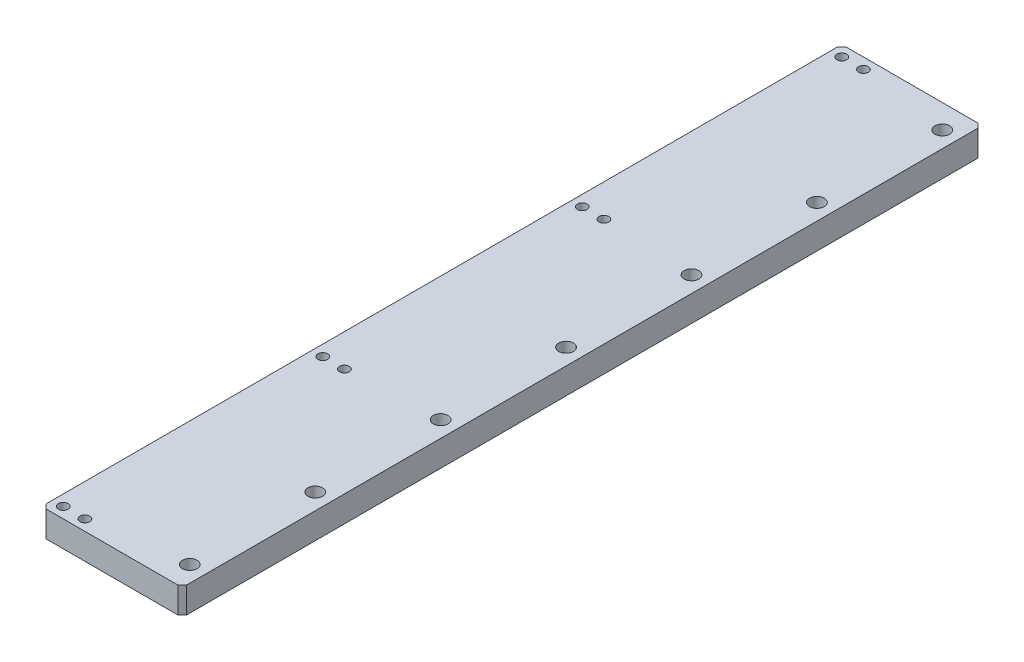
SolidWorks part; units mm, degrees
material "A6061"
ref_plane "前基準面" through (0, 0, 0) normal (0, 0, 1) x (1, 0, 0)
ref_plane "上基準面" through (0, 0, 0) normal (0, 1, 0) x (1, 0, 0)
ref_plane "右基準面" through (0, 0, 0) normal (1, 0, 0) x (0, 0, -1)
sketch "草图1" plane through (0, 0, 0) normal (0, 1, 0) x (1, 0, 0)
  line L1 (-32.5, 185) -> (32.5, 185)
  line L2 (-32.5, 185) -> (-32.5, -185)
  line L3 (-32.5, -185) -> (32.5, -185)
  line L4 (32.5, 185) -> (32.5, -185)
  line L5 (-32.5, 185) -> (32.5, -185) construction
  line L6 (-32.5, -185) -> (32.5, 185) construction
  point P0 (0, 0)
  dimension "D1" = 370
  dimension "D2" = 65
extrude "凸台-拉伸1" add sketch "草图1" along normal blind 12
hole_wizard "M8 螺纹孔1" positions "草图3" profile "草图5" tap size "M8" standard "GB" end condition through all
sketch "草图3" plane through (0, 12, 0) normal (0, 1, 0) x (1, 0, 0)
  line L1 (32.5, 185) -> (-32.5, 185) construction
  line L3 (32.5, -185) -> (32.5, 185) construction
  point P0 (25, -174)
  point P12 (25, -116)
  point P13 (25, -58)
  point P14 (25, 0)
  point P15 (25, 58)
  point P16 (25, 116)
  point P17 (25, 174)
  dimension "D2" = 11
  dimension "D3" = 7.5
  dimension "D1" = 7
sketch "草图5" plane through (25, 12, 174) normal (1, 0, 0) x (0, 0, 1)
  line L0 (0, 0) -> (0, 12)
  line L1 (0, 12) -> (3.4, 12)
  line L2 (3.4, 12) -> (3.4, 0)
  line L5 (3.4, 0) -> (0, 0)
  line L11 (0, -6.35) -> (0, 107.95) construction
  dimension "通孔螺纹孔钻头直径" = 6.8
  dimension "通孔螺纹孔钻头深度" = 12
cosmetic thread "孔螺蚊线1" parameters "D2"=8
cosmetic thread "孔螺蚊线2" parameters "D2"=8
cosmetic thread "孔螺蚊线3" parameters "D2"=8
cosmetic thread "孔螺蚊线4" parameters "D2"=8
cosmetic thread "孔螺蚊线5" parameters "D2"=8
cosmetic thread "孔螺蚊线6" parameters "D2"=8
cosmetic thread "孔螺蚊线7" parameters "D2"=8
hole_wizard "打孔尺寸(%根据)内六角圆柱头螺钉的类型1" positions "草图6" profile "草图7" counterbore size "M4" standard "GB" end condition through all
sketch "草图6" plane through (0, 0, 0) normal (0, -1, 0) x (-1, 0, 0)
  line L0 (0, 0) -> (34.7244, 0) construction
  line L2 (32.5, 185) -> (32.5, -185) construction
  point P0 (27.5, -180)
  point P6 (27.5, -60)
  point P7 (27.5, 60)
  point P15 (27.5, 180)
  dimension "D2" = 120
  dimension "D3" = 5
  dimension "D1" = 4
sketch "草图7" plane through (-27.5, 0, 180) normal (1, 0, 0) x (0, 0, -1)
  line L0 (0, 0) -> (0, 12)
  line L1 (0, 12) -> (2.25, 12)
  line L3 (2.25, 12) -> (2.25, 4.6)
  line L4 (2.25, 4.6) -> (4, 4.6)
  line L5 (4, 4.6) -> (4, 0)
  line L7 (4, 0) -> (0, 0)
  line L11 (0, -6.35) -> (0, 107.95) construction
  dimension "通孔孔直径" = 4.5
  dimension "通孔孔深度" = 12
  dimension "柱形沉头孔直径" = 8
  dimension "柱形沉头孔深度" = 4.6
chamfer "倒角1" distance 2 angle 45 4 edges at (-32.5, 6, -185) (32.5, 6, -185) (-32.5, 6, 185) (32.5, 6, 185)
pattern_linear "阵列(线性)1" count 2 spacing 10 along (1, 0, 0) of "打孔尺寸(%根据)内六角圆柱头螺钉的类型1"
